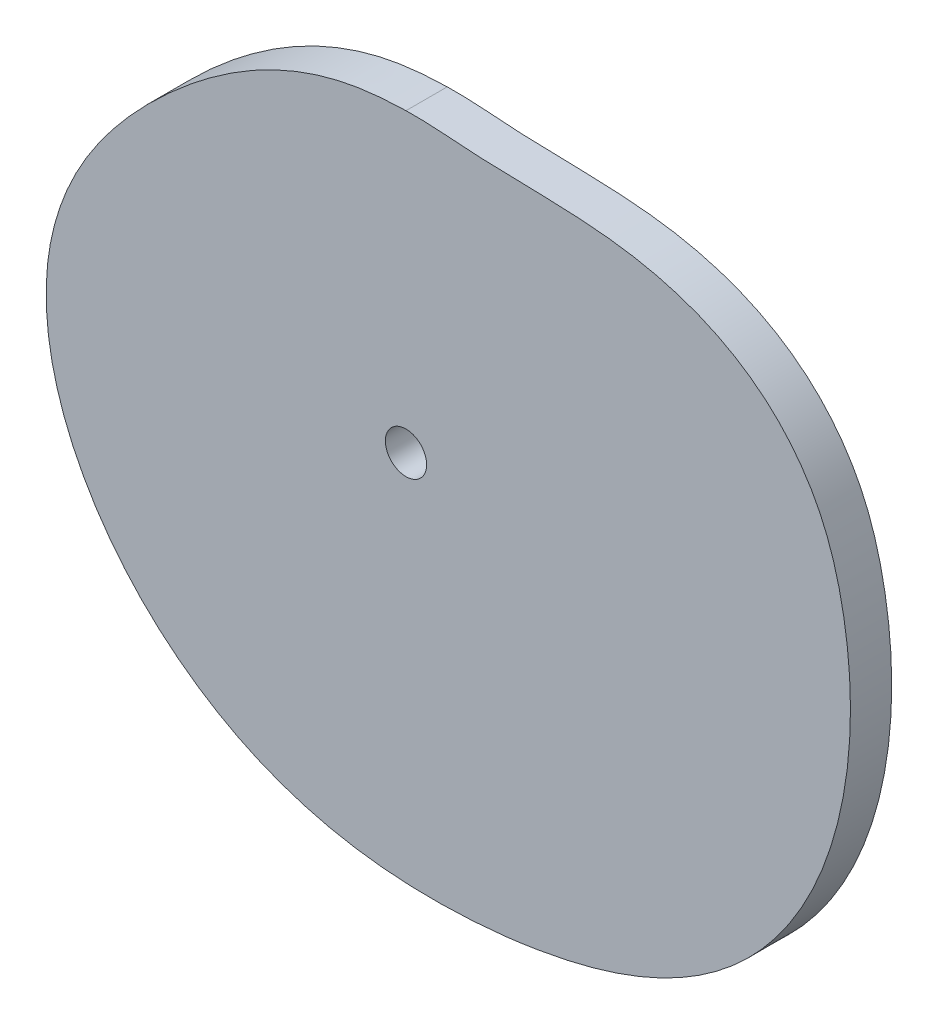
SolidWorks part; units mm, degrees
ref_plane "Front Plane" through (0, 0, 0) normal (0, 0, 1) x (1, 0, 0)
ref_plane "Top Plane" through (0, 0, 0) normal (0, 1, 0) x (1, 0, 0)
ref_plane "Right Plane" through (0, 0, 0) normal (1, 0, 0) x (0, 0, -1)
other "Configuration Table"
sketch "Sketch3" plane through (0, 0, 0) normal (0, 0, 1) x (1, 0, 0)
  circle A0 centre (0, 0) radius 5
  spline S0 degree 3 poles (32.099, -88.3151) (24.7903, -89.5442) (8.555, -91.0915) (-15.2731, -89.5787) (-40.0238, -81.711) (-60.946, -67.6391) (-77.3682, -47.6775) (-86.9267, -25.3213) (-88.0053, -2.6556) (-82.1488, 15.8763) (-73.1697, 30.3912) (-62.472, 42.4481) (-50.147, 53.3915) (-34.7459, 63.8723) (-17.4834, 70.6274) (-4.8585, 71.7045) (0, 71.8161) knots 279.040236 279.040236 279.040236 279.040236 301.306935 327.990454 350.233782 378.703779 402.465796 427.140802 450.561564 469.03891 484.738658 501.583093 517.349838 534.207201 557.456049 572.073062 572.073062 572.073062 572.073062 weights 1 1 1 1 1 1 1 1 1 1 1 1 1 1 1 1 1
  spline S1 degree 3 poles (0, 71.8161) (5.5315, 71.9431) (16.923, 70.7484) (35.3517, 70.6477) (54.6122, 69.5671) (73.2019, 64.3661) (89.3575, 54.264) (101.1461, 38.7086) (106.3085, 20.3933) (108.2587, 1.4159) (106.7756, -19.5727) (99.8723, -42.3577) (87.0064, -61.8533) (70.5817, -75.4049) (52.3526, -83.9652) (39.092, -87.139) (32.099, -88.3151) knots 0 0 0 0 16.641703 34.322343 55.462543 74.476916 91.729366 111.905407 131.542163 148.207146 169.164436 194.407337 218.993052 238.231698 257.73542 279.040236 279.040236 279.040236 279.040236 weights 1 1 1 1 1 1 1 1 1 1 1 1 1 1 1 1 1
extrude "Boss-Extrude1" add sketch "Sketch3" along normal blind 10
